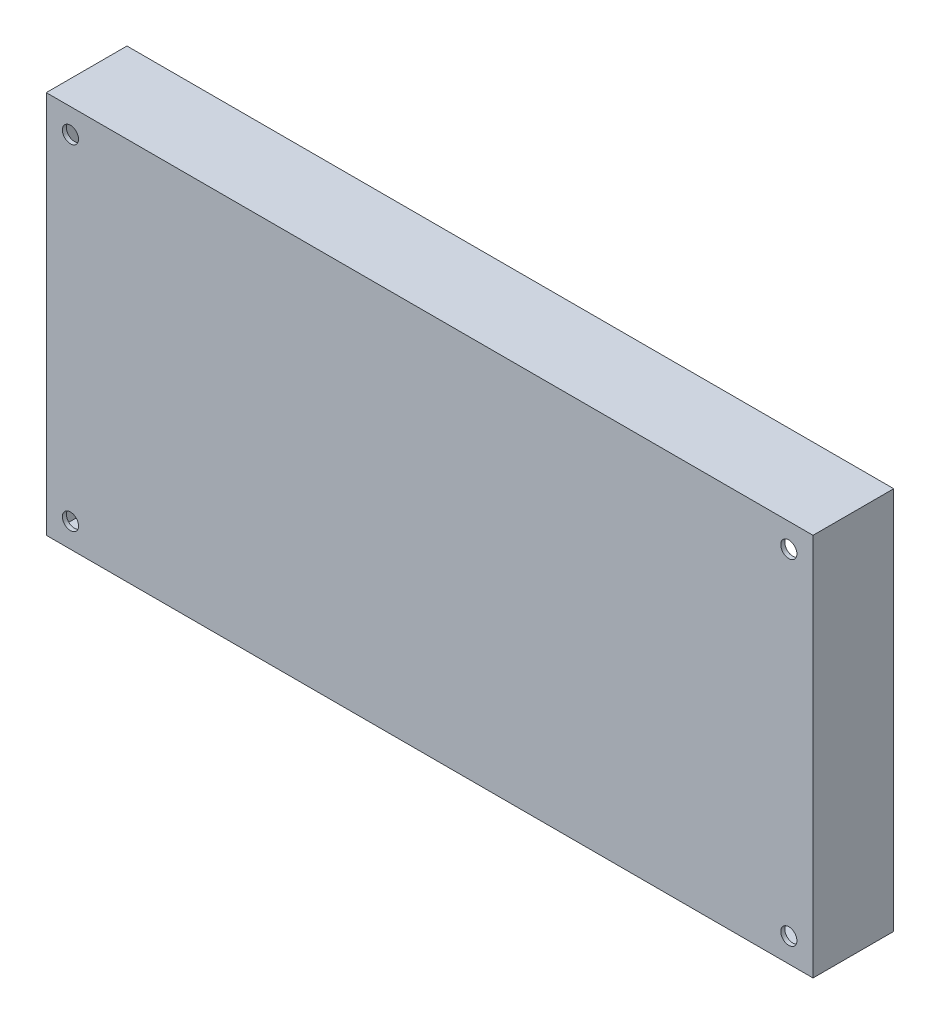
from build123d import *

# Parameters (mm, degrees)
SKETCH1_W           = 190
SKETCH1_H           = 95
BOSS_EXTRUDE1_DEPTH = 20
SHELL1_T            = -1
SKETCH2_W           = 146
SKETCH2_H           = 10
CUT_EXTRUDE1_DEPTH  = 1
SKETCH4_R           = 3.5
SKETCH4_W           = 9
SKETCH4_H           = 5.067595116
CUT_EXTRUDE2_DEPTH  = 10
SKETCH5_W           = 3
SKETCH5_H           = 2
CUT_EXTRUDE3_DEPTH  = 1
SKETCH6_R           = 2
CUT_EXTRUDE4_DEPTH  = 1
SKETCH8_W           = 3
SKETCH8_H           = 2
SKETCH8_W_2         = 27
SKETCH8_W_3         = 7
SKETCH8_W_4         = 17
SKETCH8_W_5         = 10
CUT_EXTRUDE5_DEPTH  = 1
SKETCH9_W           = 3
SKETCH9_H           = 2
SKETCH9_W_2         = 17
SKETCH9_W_3         = 6
SKETCH9_W_4         = 14
CUT_EXTRUDE6_DEPTH  = 1
SKETCH10_W          = 146
SKETCH10_H          = 12
BOSS_EXTRUDE2_DEPTH = 1
SKETCH11_R          = 3.5
SKETCH11_W          = 156
SKETCH11_H          = 11.148334169
SKETCH11_W_2        = 9
SKETCH11_H_2        = 5.067595116
BOSS_EXTRUDE3_DEPTH = 1
SKETCH12_W          = 22.5
SKETCH12_H          = 11
BOSS_EXTRUDE4_DEPTH = 1


with BuildPart() as part:
    # Sketch1 → Boss-Extrude1 (new body)
    with BuildSketch(Plane.XY):
        with Locations((67.138623448, 38.125260091)):
            Rectangle(SKETCH1_W, SKETCH1_H)
    extrude(amount=BOSS_EXTRUDE1_DEPTH)

    # Shell1
    shell1_openings = [part.faces().sort_by_distance(p)[0] for p in [
        (67.138623448, 38.125260091, 0),
    ]]
    offset(amount=SHELL1_T, openings=shell1_openings, kind=Kind.INTERSECTION)

    # Sketch2 → Cut-Extrude1 (cut)
    with BuildSketch(Plane(origin=(0, 85.625260091, 0), x_dir=(1, 0, 0), z_dir=(0, 1, 0))):
        Polygon((139.138623448, -9), (139.138623448, -8), (139.638623448, -8), (149.638623448, -8), (149.638623448, -19), (139.638623448, -19), (139.138623448, -19), (127.138623448, -19), (127.138623448, -9), align=None)
        with Locations((53.138623448, -14)):
            Rectangle(SKETCH2_W, SKETCH2_H)
    extrude(amount=-CUT_EXTRUDE1_DEPTH, mode=Mode.SUBTRACT)

    # Sketch4 → Cut-Extrude2 (cut)
    with BuildSketch(Plane.XZ.offset(9.374739909)):
        with Locations(Location((144.138623448, 6.5, 0), (0, 0, 270))):
            Circle(SKETCH4_R)
        Polygon((124.166122212, 9.851665831), (138.166122212, 9.851665831), (138.166122212, 19), (-17.833877788, 19), (-17.833877788, 9.851665831), (-14.833877788, 9.851665831), (-14.833877788, 7.851665831), (-11.833877788, 7.851665831), (-11.833877788, 9.851665831), (5.166122212, 9.851665831), (5.166122212, 7.851665831), (8.166122212, 7.851665831), (8.166122212, 9.851665831), (14.166122212, 9.851665831), (14.166122212, 7.851665831), (17.166122212, 7.851665831), (17.166122212, 9.851665831), (34.166122212, 9.851665831), (34.166122212, 7.851665831), (37.166122212, 7.851665831), (37.166122212, 9.851665831), (43.166122212, 9.851665831), (43.166122212, 7.851665831), (46.166122212, 7.851665831), (46.166122212, 9.851665831), (63.166122212, 9.851665831), (63.166122212, 7.851665831), (66.166122212, 7.851665831), (66.166122212, 9.851665831), (72.166122212, 9.851665831), (72.166122212, 7.851665831), (75.166122212, 7.851665831), (75.166122212, 9.851665831), (92.166122212, 9.851665831), (92.166122212, 7.851665831), (95.166122212, 7.851665831), (95.166122212, 9.851665831), (101.166122212, 9.851665831), (101.166122212, 7.851665831), (104.166122212, 7.851665831), (104.166122212, 9.851665831), (121.166122212, 9.851665831), (121.166122212, 7.851665831), (124.166122212, 7.851665831), align=None)
        with Locations((109.666122212, 4.317868273)):
            Rectangle(SKETCH4_W, SKETCH4_H)
    extrude(amount=-CUT_EXTRUDE2_DEPTH, mode=Mode.SUBTRACT)

    # Sketch5 → Cut-Extrude3 (cut)
    with BuildSketch(Plane(origin=(0, 85.625260091, 0), x_dir=(1, 0, 0), z_dir=(0, 1, 0))):
        with Locations((-15.361376552, -8)):
            Rectangle(SKETCH5_W, SKETCH5_H)
        with Locations((14.638623448, -8)):
            Rectangle(SKETCH5_W, SKETCH5_H)
        with Locations((24.638623448, -8)):
            Rectangle(SKETCH5_W, SKETCH5_H)
        with Locations((54.638623448, -8)):
            Rectangle(SKETCH5_W, SKETCH5_H)
        with Locations((64.638623448, -8)):
            Rectangle(SKETCH5_W, SKETCH5_H)
        with Locations((84.638623448, -8)):
            Rectangle(SKETCH5_W, SKETCH5_H)
        with Locations((94.638623448, -8)):
            Rectangle(SKETCH5_W, SKETCH5_H)
        with Locations((114.638623448, -8)):
            Rectangle(SKETCH5_W, SKETCH5_H)
    extrude(amount=-CUT_EXTRUDE3_DEPTH, mode=Mode.SUBTRACT)

    # Sketch6 → Cut-Extrude4 (cut)
    with BuildSketch(Plane.XY.offset(20)):
        with Locations((-21.861376552, -3.374739909)):
            Circle(SKETCH6_R)
        with Locations((-21.861376552, 79.625260091)):
            Circle(SKETCH6_R)
        with Locations((156.138623448, 79.625260091)):
            Circle(SKETCH6_R)
        with Locations((156.138623448, -3.374739909)):
            Circle(SKETCH6_R)
    extrude(amount=-CUT_EXTRUDE4_DEPTH, mode=Mode.SUBTRACT)

    # Sketch8 → Cut-Extrude5 (cut)
    with BuildSketch(Plane(origin=(0, 85.625260091, 0), x_dir=(1, 0, 0), z_dir=(0, 1, 0))):
        with Locations((-18.361376552, -8)):
            Rectangle(SKETCH8_W, SKETCH8_H)
        with Locations((-0.361376552, -8)):
            Rectangle(SKETCH8_W_2, SKETCH8_H)
        with Locations((19.638623448, -8)):
            Rectangle(SKETCH8_W_3, SKETCH8_H)
        with Locations((39.638623448, -8)):
            Rectangle(SKETCH8_W_2, SKETCH8_H)
        with Locations((59.638623448, -8)):
            Rectangle(SKETCH8_W_3, SKETCH8_H)
        with Locations((74.638623448, -8)):
            Rectangle(SKETCH8_W_4, SKETCH8_H)
        with Locations((89.638623448, -8)):
            Rectangle(SKETCH8_W_3, SKETCH8_H)
        with Locations((104.638623448, -8)):
            Rectangle(SKETCH8_W_4, SKETCH8_H)
        with Locations((121.138623448, -8)):
            Rectangle(SKETCH8_W_5, SKETCH8_H)
    extrude(amount=-CUT_EXTRUDE5_DEPTH, mode=Mode.SUBTRACT)

    # Sketch9 → Cut-Extrude6 (cut)
    with BuildSketch(Plane.XZ.offset(9.374739909)):
        with Locations((-16.333877788, 8.851665831)):
            Rectangle(SKETCH9_W, SKETCH9_H)
        with Locations((-3.333877788, 8.851665831)):
            Rectangle(SKETCH9_W_2, SKETCH9_H)
        with Locations((11.166122212, 8.851665831)):
            Rectangle(SKETCH9_W_3, SKETCH9_H)
        with Locations((25.666122212, 8.851665831)):
            Rectangle(SKETCH9_W_2, SKETCH9_H)
        with Locations((40.166122212, 8.851665831)):
            Rectangle(SKETCH9_W_3, SKETCH9_H)
        with Locations((54.666122212, 8.851665831)):
            Rectangle(SKETCH9_W_2, SKETCH9_H)
        with Locations((69.166122212, 8.851665831)):
            Rectangle(SKETCH9_W_3, SKETCH9_H)
        with Locations((83.666122212, 8.851665831)):
            Rectangle(SKETCH9_W_2, SKETCH9_H)
        with Locations((98.166122212, 8.851665831)):
            Rectangle(SKETCH9_W_3, SKETCH9_H)
        with Locations((112.666122212, 8.851665831)):
            Rectangle(SKETCH9_W_2, SKETCH9_H)
        with Locations((131.166122212, 8.851665831)):
            Rectangle(SKETCH9_W_4, SKETCH9_H)
    extrude(amount=-CUT_EXTRUDE6_DEPTH, mode=Mode.SUBTRACT)

    # Sketch10 → Boss-Extrude2 (add)
    with BuildSketch(Plane(origin=(0, 85.625260091, 0), x_dir=(1, 0, 0), z_dir=(0, 1, 0))):
        with Locations((53.138623448, -13)):
            Rectangle(SKETCH10_W, SKETCH10_H)
    extrude(amount=-BOSS_EXTRUDE2_DEPTH)

    # Sketch11 → Boss-Extrude3 (add)
    with BuildSketch(Plane.XZ.offset(9.374739909)):
        with Locations((144.138623448, 6.5)):
            Circle(SKETCH11_R)
        with Locations((60.166122212, 13.425832916)):
            Rectangle(SKETCH11_W, SKETCH11_H)
        with Locations((109.666122212, 4.317868273)):
            Rectangle(SKETCH11_W_2, SKETCH11_H_2)
    extrude(amount=-BOSS_EXTRUDE3_DEPTH)

    # Sketch12 → Boss-Extrude4 (add)
    with BuildSketch(Plane(origin=(0, 85.625260091, 0), x_dir=(1, 0, 0), z_dir=(0, 1, 0))):
        with Locations((138.388623448, -13.5)):
            Rectangle(SKETCH12_W, SKETCH12_H)
    extrude(amount=-BOSS_EXTRUDE4_DEPTH)


solid = part.part
